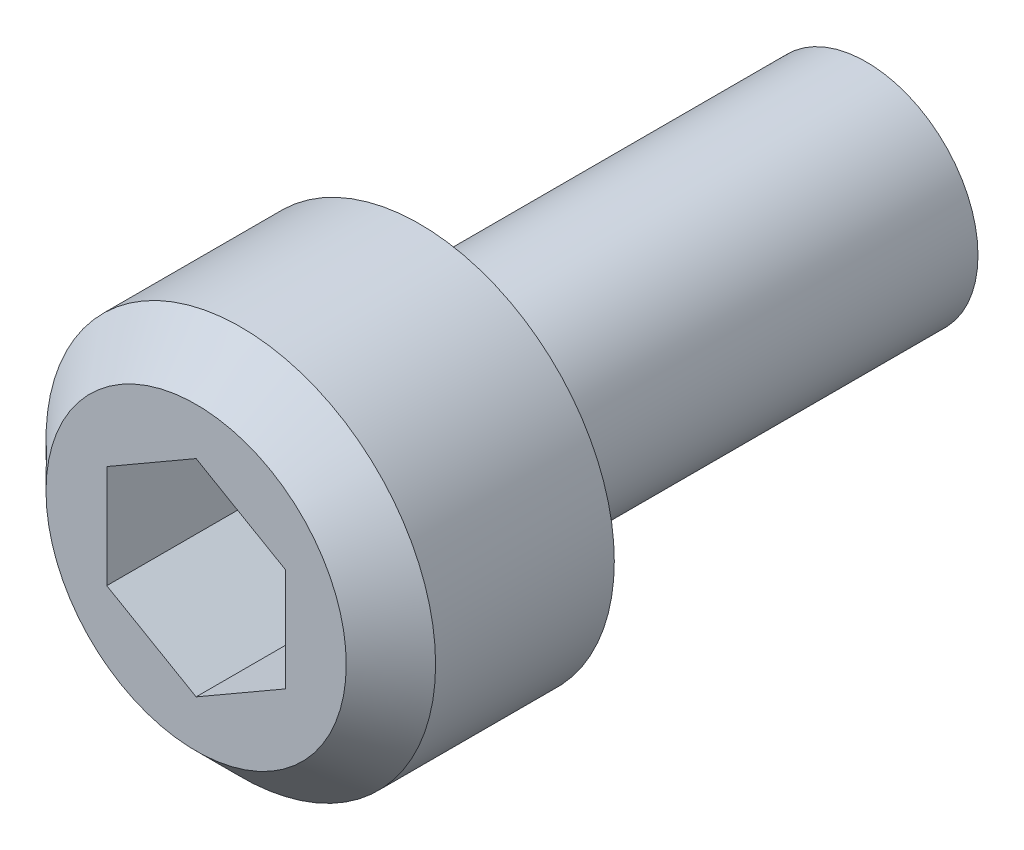
from build123d import *

# Parameters (mm, degrees)
SKETCH_1_R          = 4.36
EXTRUDE_1_DEPTH     = 5
CUT_EXTRUDE_1_DEPTH = 4
CHAMFER_1_SIZE      = 1
SKETCH_3_R          = 2.5
EXTRUDE_2_DEPTH     = 10


with BuildPart() as part:
    # 草图1 → 凸台-拉伸1 (new body)
    with BuildSketch(Plane.XY):
        Circle(SKETCH_1_R)
    extrude(amount=EXTRUDE_1_DEPTH)

    # 草图2 → 切除-拉伸1 (cut)
    with BuildSketch(Plane.XY.offset(5)):
        Polygon((0, 2.309401077), (-2, 1.154700538), (-2, -1.154700538), (0, -2.309401077), (2, -1.154700538), (2, 1.154700538), align=None)
    extrude(amount=-CUT_EXTRUDE_1_DEPTH, mode=Mode.SUBTRACT)

    # 倒角1
    chamfer_1_edges = [part.edges().sort_by_distance(p)[0] for p in [
        (-4.36, 0, 5),
    ]]
    chamfer(chamfer_1_edges, length=CHAMFER_1_SIZE)

    # 草图3 → 凸台-拉伸2 (add)
    with BuildSketch(Plane(origin=(0, 0, 0), x_dir=(-1, 0, 0), z_dir=(0, 0, -1))):
        with Locations(Location((0, 0, 0), (0, 0, 180))):
            Circle(SKETCH_3_R)
    extrude(amount=EXTRUDE_2_DEPTH)


solid = part.part
